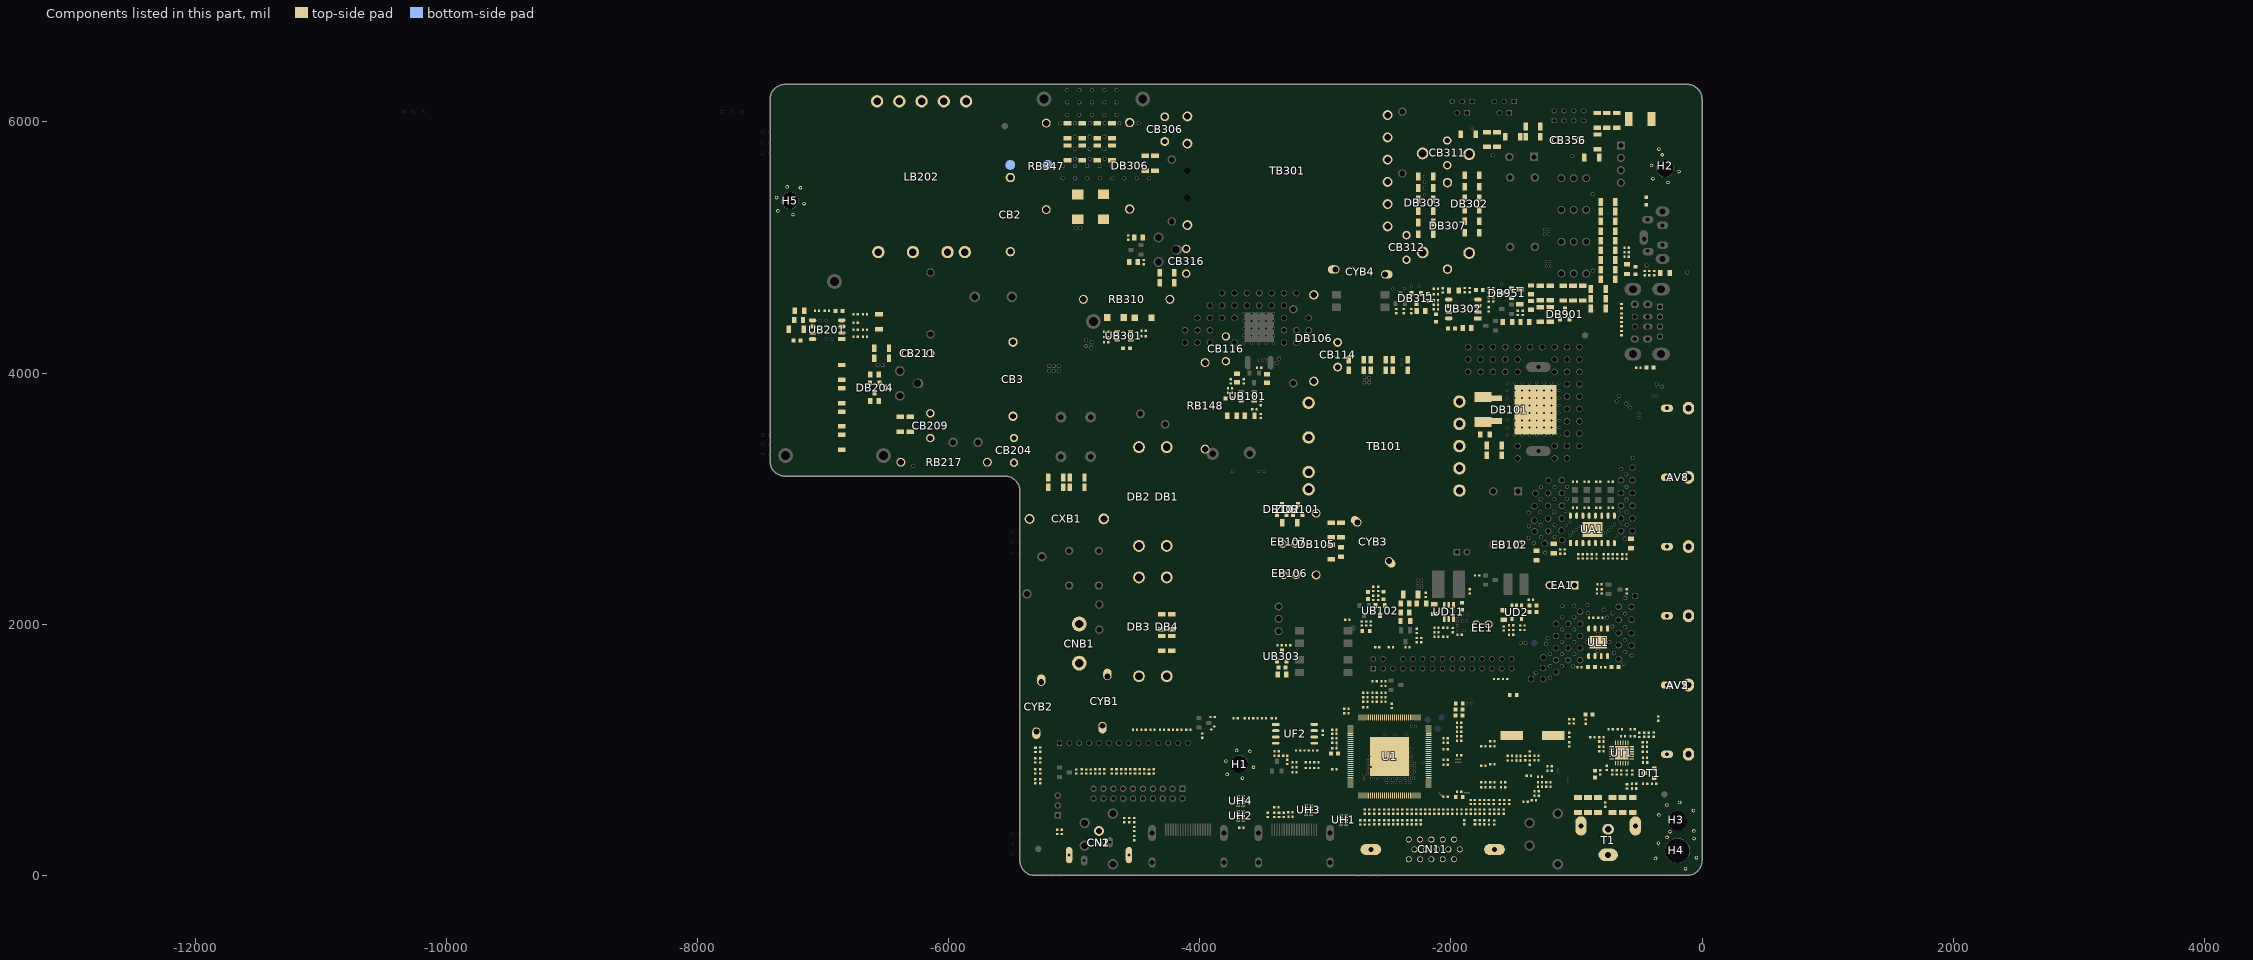
[diagram p0: the components of this part, seen from the top]
# Altium PCB MISC84277.PcbDoc (part 3 of 15)
Units mil, origin at the board's own origin, x right, y up, seen from the top; angles counter-clockwise.
Board outline 7422.08 x 6299.21 mil, 2 copper layers (TopLayer, BottomLayer), stack 61.855 mil thick; 709 components, 395 nets, 2812 pads, 811 vias.

## Components (designator, comment, footprint, x,y, rotation, side; value= is the part's Value field where it differs from the comment) (continued)
RB210 "10ohm-1206-±5%-1/4W" R1206 -7213.93,4349.5 r180 top
RB212 "47ohm-0805-±5%-1/8W" R0805 -6589.92,3989.81 r0 top
RB213 "20ohm-0805-±5%-1/8W" R0805 -6589.92,3777.97 r0 top
RB214 "10Kohm-0402-±5%-1/16W" R0402 -6502.12,3881.88 r90 top
RB215 "510ohm-0402-±5%-1/16W" R0402 -6666.39,4468.8 r0 top
RB217 "MOF-0R1ohm-±5%-2WS (tape and reel/Futaba)" R2-H-17.5 -6036.5,3290.5 r180 top
RB218 "1R6ohm-1206-±1%-1/4W" R1206 -6555,4409.94 r90 top
RB219 "22ohm-1206-±5%-1/4W" R1206 -6305.64,3592.04 r90 top
RB220 "22ohm-1206-±5%-1/4W" R1206 -6385.37,3592.04 r90 top
RB221 "1Kohm-0402-±5%-1/16W" R0402 -6666.39,4345.31 r180 top
RB223 "22ohm-1206-±5%-1/4W" R1206 -6534.37,4118.08 r180 top
RB224 "22ohm-1206-±5%-1/4W" R1206 -6534.37,4196.82 r180 top
RB225 "10Kohm-0402-±5%-1/16W" R0402 -6970.22,4496.35 r180 top
RB226 "47Kohm-0402-±1%-1/16W" R0402 -6741.19,4400.61 r180 top
RB227 "NC/0ohm-0402-±5%-1/16W" R0402 -7048.96,4496.35 r0 top
RB301 "47ohm-0805-±5%-1/8W" R0805 -1871,4360.5 r0 top
RB302 "8K2ohm-0402-±1%-1/16W" R0402 -3296.5,1832.5 r0 top
RB303 "NC/10Kohm-0402-±5%-1/16W" R0402 -4745.41,4244.24 r180 top
RB304 "47Kohm-0402-±1%-1/16W" R0402 -4447.08,4338.63 r0 top
RB305 "510ohm-0402-±5%-1/16W" R0402 -4745.41,4330.86 r180 top
RB306 "47ohm-0805-±5%-1/8W" R0805 -4489.97,5079.5 r0 top
RB307 "510ohm-0402-±5%-1/16W" R0402 -4569.47,5079.5 r270 top
RB308 "20ohm-0805-±5%-1/8W" R0805 -4527.5,4883.5 r0 top
RB309 "10Kohm-0402-±5%-1/16W" R0402 -4448,4883.5 r90 top
RB310 "MOF-0R22ohm-±5%-2WS (tape and reel/Futaba)" R2-H-17.5 -4582.61,4587.13 r180 top
RB314 "10ohm-1206-±5%-1/4W" R1206 -4435.6,5670.34 r270 top
RB315 "10ohm-1206-±5%-1/4W" R1206 -4356.88,5670.34 r270 top
RB317 "330Kohm-1206-±5%-1/4W" R1206 -4699.09,5753.57 r270 top
RB318 "330Kohm-1206-±5%-1/4W" R1206 -4817.2,5753.57 r270 top
RB319 "330Kohm-1206-±5%-1/4W" R1206 -4935.31,5753.57 r270 top
RB320 "330Kohm-1206-±5%-1/4W" R1206 -5053.42,5753.57 r270 top
RB321 "330Kohm-1206-±5%-1/4W" R1206 -5053.42,5930.74 r270 top
RB322 "330Kohm-1206-±5%-1/4W" R1206 -4699.09,5930.74 r270 top
RB323 "330Kohm-1206-±5%-1/4W" R1206 -4817.2,5930.74 r270 top
RB324 "330Kohm-1206-±5%-1/4W" R1206 -4935.31,5930.74 r270 top
RB325 "49K9ohm-0402-±1%-1/16W" R0402 -3364,1832.5 r180 top
RB326 "100ohm-0805-±5%-1/8W" R0805 -3345.5,1600 r0 top
RB328 "270Kohm-1206-±5%-1/4W" R1206 -1832.22,5484.11 r180 top
RB329 "270Kohm-1206-±5%-1/4W" R1206 -1832.22,5392.31 r0 top
RB330 "270Kohm-1206-±5%-1/4W" R1206 -1832.22,5116.9 r180 top
RB331 "270Kohm-1206-±5%-1/4W" R1206 -2200.06,5198.86 r180 top
RB332 "NC/270Kohm-1206-±5%-1/4W" R1206 -1832.22,5575.91 r180 top
RB333 "NC/270Kohm-1206-±5%-1/4W" R1206 -1832.22,5300.5 r0 top
RB334 "NC/270Kohm-1206-±5%-1/4W" R1206 -1832.22,5208.7 r180 top
RB335 "NC/270Kohm-1206-±5%-1/4W" R1206 -2200.06,5107.06 r180 top
RB337 "1R6ohm-1206-±1%-1/4W" R1206 -879.7,5717.5 r0 top
RB338 "1R6ohm-1206-±1%-1/4W" R1206 -833.45,5841.2 r270 top
RB339 "1R6ohm-1206-±1%-1/4W" R1206 -680.42,6012.54 r90 top
RB340 "1R6ohm-1206-±1%-1/4W" R1206 -758.2,6012.55 r90 top
RB341 "2R2ohm-1206-±1%-1/4W" R1206 -835.79,6012.54 r90 top
RB345 "5K6ohm-0402-±1%-1/16W" R0402 -2065.5,4659 r270 top
RB346 "510ohm-0402-±5%-1/16W" R0402 -2435,4493.5 r90 top
RB347 "NC/MOF-300Kohm-±5%-2WS (tape and reel/Futaba)" R2-H-17.5 -5223,5646.5 r270 top
RB348 "1Kohm-0402-±5%-1/16W" R0402 -2120.5,4508 r0 top
RB349 "27Kohm-0402-±1%-1/16W" R0402 -2120.5,4544.5 r180 top
RB350 "1Kohm-0603-±1%-1/10W" R0603 -2119.5,4437.5 r270 top
RB351 "10Kohm-0402-±5%-1/16W" R0402 -2120.57,4673.43 r0 top
RB352 "NC/20Kohm-0402-±1%-1/16W" R0402 -1850.5,4660.5 r270 top
RB354 "3Kohm-0402-±1%-1/16W" R0402 -1700,4507 r270 top
RB355 "4K7ohm-0402-±1%-1/16W" R0402 -1662.85,4587.77 r90 top
RB356 "2M2ohm-0402-±5%-1/16W" R0402 -2318,4493.5 r270 top
RB357 "3Kohm-0402-±1%-1/16W" R0402 -1699.45,4658.94 r90 top
RB358 "120Kohm-0805-±5%-1/8W" R0805 -1363,4663.5 r270 top (schematic designator RB364)
RB359 "120Kohm-0805-±5%-1/8W" R0805 -1363,4540 r270 top
RB360 "150Kohm-1206-±5%-1/4W" R1206 -1288.48,4637.59 r90 top
RB361 "150Kohm-1206-±5%-1/4W" R1206 -1209.74,4466.73 r90 top
RB362 "150Kohm-1206-±5%-1/4W" R1206 -1288.48,4466.73 r90 top
RB363 "150Kohm-1206-±5%-1/4W" R1206 -1209.74,4637.59 r90 top
RB364 "30Kohm-0805-±1%-1/8W" R0805 -1412,4407.5 r180 top
RB365 "10ohm-0805-±5%-1/8W" R0805 -2237.5,4493 r0 top
RB366 "47Kohm-0402-±1%-1/16W" R0402 -1889,4660.5 r270 top
RB367 "1Kohm-0402-±5%-1/16W" R0402 -1662.84,4658.94 r90 top
RB368 "68ohm-1206-±5%-1/4W" R1206 -2200.06,5290.66 r180 top
RB369 "68ohm-1206-±5%-1/4W" R1206 -2200.06,5382.46 r180 top
RB370 "68ohm-1206-±5%-1/4W" R1206 -2200.06,5474.26 r180 top
RB371 "68ohm-1206-±5%-1/4W" R1206 -2200.06,5566.07 r180 top
RB384 "1Kohm-0603-±1%-1/10W" R0603 -2675.28,1944.88 r180 top
RB385 "4K7ohm-0402-±1%-1/16W" R0402 -2675.28,2005.98 r90 top
RB386 "9K1ohm-0402-±1%-1/16W" R0402 -2711.79,2005.98 r270 top
RB391 "22ohm-1206-±5%-1/4W" R1206 -4261.46,4798.93 r180 top
RB392 "22ohm-1206-±5%-1/4W" R1206 -4261.32,4720.7 r180 top
RB901 "NC/470ohm-1206-±5%-1/4W" R1206 -1028.31,4637.19 r270 top
RB902 "NC/470ohm-1206-±5%-1/4W" R1206 -1105.54,4637.19 r270 top
RB903 "NC/470ohm-1206-±5%-1/4W" R1206 -951.09,4637.19 r270 top
RB904 "0ohm-1206-±5%-1/4W" R1206 -1346.23,5881.2 r0 top
RB905 "NC/0ohm-1206-±5%-1/4W" R1206 -1346.23,5963.8 r0 top
RB911 "NC/10ohm-1206-±5%-1/4W" R1206 -749.28,5130.73 r180 top
RB912 "NC/10ohm-1206-±5%-1/4W" R1206 -749.28,5054.26 r180 top
RB913 "NC/10ohm-1206-±5%-1/4W" R1206 -749.28,4977.39 r180 top
RB921 "NC/10ohm-1206-±5%-1/4W" R1206 -749.28,5363.12 r180 top
RB922 "NC/10ohm-1206-±5%-1/4W" R1206 -749.28,5286.45 r180 top
RB923 "NC/10ohm-1206-±5%-1/4W" R1206 -749.28,5209.28 r180 top
RB931 "NC/10ohm-1206-±5%-1/4W" R1206 -827.49,4670.39 r180 top
RB932 "NC/10ohm-1206-±5%-1/4W" R1206 -827.49,4592.62 r180 top
RB933 "NC/10ohm-1206-±5%-1/4W" R1206 -827.49,4514.85 r180 top
RB941 "NC/10ohm-1206-±5%-1/4W" R1206 -749.28,4900.13 r180 top
RB942 "NC/10ohm-1206-±5%-1/4W" R1206 -749.18,4823.97 r180 top
RB943 "NC/10ohm-1206-±5%-1/4W" R1206 -749.28,4748.1 r180 top
RB951 "NC/2Kohm-0402-±1%-1/16W" R0402 -1469.49,4480.1 r90 top
RB952 "NC/20Kohm-1206-±5%-1/4W" R1206 -1452.6,4608.64 r90 top
RD1 "100Kohm-0402-±1%-1/16W" R0402 -2115,1973 r0 top
RD6 "12K4ohm-0402-±1%-1/16W" R0402 -1520,1954 r180 top
RD7 "13Kohm-0402-±1%-1/16W" R0402 -1520,1991 r0 top
RD8 "68Kohm-0402-±1%-1/16W" R0402 -1431,1954 r0 top
RD12 "18Kohm-0402-±1%-1/16W" R0402 -2044,1900 r0 top
RD13 "100Kohm-0402-±1%-1/16W" R0402 -2115,1936 r0 top
RD15 "22ohm-0402-±5%-1/16W" R0402 -1984.25,1952.76 r270 top
RD16 "3K3ohm-0402-±1%-1/16W" R0402 -2115,1900 r0 top
RF1 "NC/1Mohm-0402-±5%-1/16W" R0402 -1742,1026.8 r180 top
RF2 "10Kohm-0402-±5%-1/16W" R0402 -3489,1251 r180 top
RF3 "4K7ohm-0402-±5%-1/16W" R0402 -3411,1251 r180 top
RF8 "4K7ohm-0402-±5%-1/16W" R0402 -2833,1291 r180 top
RF9 "4K7ohm-0402-±5%-1/16W" R0402 -2833,1327 r180 top
RF10 "100ohm-0402-±5%-1/16W" R0402 -2572,508 r270 top
RF11 "100ohm-0402-±5%-1/16W" R0402 -2722,422 r270 top
RF12 "68ohm-0402-±5%-1/16W" R0402 -1916,507 r90 top
RF13 "4K7ohm-0402-±5%-1/16W" R0402 -2608,1381 r180 top
RF14 "200Kohm-0402-±5%-1/16W" R0402 -1291,784 r0 top
RF15 "200Kohm-0402-±5%-1/16W" R0402 -1214,870 r0 top
RF16 "68ohm-0402-±5%-1/16W" R0402 -2423,508 r90 top
RF18 "4K7ohm-0402-±5%-1/16W" R0402 -2682,1381 r180 top
RF19 "68ohm-0402-±5%-1/16W" R0402 -2168,507 r270 top
RG1 "510ohm-0402-±5%-1/16W" R0402 -2682,1417 r0 top
RG2 "0ohm-0402-±5%-1/16W" R0402 -2608,1417 r180 top
RH1 "10Kohm-0402-±5%-1/16W" R0402 -4479.9,828.18 r90 top
RH2 "10Kohm-0402-±5%-1/16W" R0402 -4441.8,828.18 r90 top
RH3 "22ohm-0402-±5%-1/16W" R0402 -4367.2,828.18 r90 top
RH4 "22ohm-0402-±5%-1/16W" R0402 -4553.4,828.18 r90 top
RH5 "1Kohm-0402-±5%-1/16W" R0402 -4867.9,827.4 r270 top
RH6 "10Kohm-0402-±5%-1/16W" R0402 -4904,826.9 r90 top
RH7 "10Kohm-0402-±5%-1/16W" R0402 -4985.1,826.9 r90 top
RH8 "10Kohm-0402-±5%-1/16W" R0402 -3139.7,899.9 r0 top
RH9 "10Kohm-0402-±5%-1/16W" R0402 -3246.3,899.9 r180 top
RH10 "22ohm-0402-±5%-1/16W" R0402 -3072.4,855.1 r180 top
RH11 "22ohm-0402-±5%-1/16W" R0402 -3072.4,899.9 r180 top
RH13 "220ohm-0402-±5%-1/16W" R0402 -3139.7,855.1 r180 top
RH14 "1Kohm-0402-±5%-1/16W" R0402 -3319.7,953.77 r0 top
RH15 "10Kohm-0402-±5%-1/16W" R0402 -3246.3,823 r0 top
RH16 "10Kohm-0402-±5%-1/16W" R0402 -3246.3,860 r0 top
RH19 "NC/NC/100ohm-0402-±5%-1/16W" R0402 -3388.3,989.7 r180 top
RH20 "NC/NC/100ohm-0402-±5%-1/16W" R0402 -3388.3,954 r180 top
RH55 "NC/33Kohm-0402-±5%-1/16W" R0402 -4795.5,828.1 r270 top
RH56 "NC/22Kohm-0402-±5%-1/16W" R0402 -4759.7,828.2 r270 top
RI1 "NC/0ohm-0402-±5%-1/16W" R0402 -1734,423 r270 top
RI2 "0ohm-0402-±5%-1/16W" R0402 -1734,507 r270 top
RI3 "33ohm-0402-±5%-1/16W" R0402 -2024,507 r270 top
RI4 "10Kohm-0402-±5%-1/16W" R0402 -1692,507 r270 top
RI5 "12Kohm-0402-±5%-1/16W" R0402 -1809,584 r270 top
RI6 "10Kohm-0402-±5%-1/16W" R0402 -1698,584 r90 top
RI7 "12Kohm-0402-±5%-1/16W" R0402 -1735,584 r90 top
RI8 "10Kohm-0402-±5%-1/16W" R0402 -1224,743 r0 top
RI9 "12Kohm-0402-±5%-1/16W" R0402 -1291,743 r0 top
RI10 "10Kohm-0402-±5%-1/16W" R0402 -1224,707 r0 top
RI11 "12Kohm-0402-±5%-1/16W" R0402 -1291,707 r180 top
RI12 "33ohm-0402-±5%-1/16W" R0402 -2242,508 r90 top
RI13 "75ohm-0402-±5%-1/16W" R0402 -2242,423 r90 top
RI14 "NC/33ohm-0402-±5%-1/16W" R0402 -2314,423 r270 top
RI15 "NC/75ohm-0402-±5%-1/16W" R0402 -2278,423 r270 top
RI16 "NC/33ohm-0402-±5%-1/16W" R0402 -2096,507 r270 top
RI17 "NC/75ohm-0402-±5%-1/16W" R0402 -1895,423 r270 top
RI18 "75ohm-0402-±5%-1/16W" R0402 -1697,422 r90 top
RK1 "22ohm-0402-±5%-1/16W" R0402 -3897.08,1173.56 r225 top
RK2 "1Kohm-0402-±5%-1/16W" R0402 -3897.5,1261.1 r0 top
RK3 "1Kohm-0402-±5%-1/16W" R0402 -3626,1251 r0 top
RK4 "4K7ohm-0402-±1%-1/16W" R0402 -3557,1251 r0 top
RK5 "510ohm-0402-±1%-1/16W" R0402 -5271.45,1001.36 r270 top
RK6 "680ohm-0402-±1%-1/16W" R0402 -5308.96,749.44 r90 top
RK7 "1Kohm-0402-±1%-1/16W" R0402 -5271.45,749.44 r90 top
RK8 "1K2ohm-0402-±1%-1/16W" R0402 -5271.45,828.18 r90 top
RK9 "2K2ohm-0402-±1%-1/16W" R0402 -5308.96,828.18 r90 top
RK10 "4K7ohm-0402-±1%-1/16W" R0402 -5271.45,916.17 r90 top
RK11 "15Kohm-0402-±1%-1/16W" R0402 -5308.96,916.17 r90 top
RK15 "4K7ohm-0402-±5%-1/16W" R0402 -4516.1,1160 r0 top
RK16 "1Kohm-0402-±5%-1/16W" R0402 -4448.3,1160 r180 top
RK18 "33Kohm-0402-±5%-1/16W" R0402 -2537,1381 r0 top
RK20 "10Kohm-0402-±5%-1/16W" R0402 -4162.6,1160 r180 top
RK21 "510ohm-0402-±5%-1/16W" R0402 -4230.6,1160 r180 top
RM1 "4K7ohm-0402-±5%-1/16W" R0402 -837,2262 r270 top
RM2 "200Kohm-0402-±1%-1/16W" R0402 -817,2317 r0 top
RM3 "10Kohm-0402-±5%-1/16W" R0402 -2537,1417 r180 top
RM4 "4K7ohm-0402-±5%-1/16W" R0402 -1791,2388 r180 top
RM5 "4K7ohm-0402-±5%-1/16W" R0402 -2235,1874 r90 top
RM6 "NC/4K7ohm-0402-±5%-1/16W" R0402 -2478,1817 r0 top
RM7 "47Kohm-0402-±1%-1/16W" R0402 -2272,1874 r90 top
RM8 "4K7ohm-0402-±5%-1/16W" R0402 -2608,1545 r0 top
RM10 "2K2ohm-0402-±5%-1/16W" R0402 -2537,1545 r0 top
RO1 "NC/510ohm-0402-±5%-1/16W" R0402 -1537,584 r270 top
RO2 "NC/0ohm-0402-±5%-1/16W" R0402 -1771,507 r90 top
RO3 "NC/47Kohm-0402-±5%-1/16W" R0402 -4522.89,369.5 r270 top
RO5 "NC/510ohm-0402-±5%-1/16W" R0402 -1581,508 r270 top
RO6 "0ohm-0402-±5%-1/16W" R0402 -4603.2,439.7 r90 top
RO7 "NC/47Kohm-0402-±5%-1/16W" R0402 -4563.06,439.7 r90 top
RO9 "NC/220ohm-0402-±5%-1/16W" R0402 -3150,994.42 r180 top
RO10 "NC/100ohm-0402-±5%-1/16W" R0402 -3217.4,994.42 r180 top
RO12 "75ohm-0402-±5%-1/16W" R0402 -1844,507 r270 top
RO13 "0ohm-0402-±5%-1/16W" R0402 -1808,507 r90 top
RO15 "NC/0ohm-0402-±5%-1/16W" R0402 -1655,507 r90 top
RO16 "NC/0ohm-0402-±5%-1/16W" R0402 -1771,423 r270 top
RO17 "NC/0ohm-0402-±5%-1/16W" R0402 -1610,584 r270 top
RT1 "0ohm-0402-±5%-1/16W" L0402 -1462.17,951.3 r180 top
RT2 "100ohm-0402-±5%-1/16W" R0402 -802.35,1025.41 r0 top
RT3 "4K7ohm-0402-±5%-1/16W" R0402 -1059.05,1227.1 r270 top
RT4 "4K7ohm-0402-±5%-1/16W" R0402 -1021.7,1227.1 r270 top
RT5 "33ohm-0402-±5%-1/16W" R0402 -422.97,1119.86 r270 top
RT6 "33ohm-0402-±5%-1/16W" R0402 -385.62,1120.41 r270 top
RT7 "FCM1005KF-121T06(120ohm-500mA)" R0402 -928.4,1224.4 r270 top
RT9 "220ohm-0402-±5%-1/16W" R0402 -1318.94,950.79 r0 top
RT10 "220ohm-0402-±5%-1/16W" R0402 -1318.94,915.79 r0 top
RT11 "1K8ohm-0402-±5%-1/16W" R0402 -552.92,1107.68 r180 top
RT12 "430ohm-0402-±5%-1/16W" R0402 -1409.45,933.07 r90 top
RT14 "0ohm-0402-±5%-1/16W" L0402 -1462.17,914.8 r180 top
RT18 "10Kohm-0402-±5%-1/16W" R0402 -1670,885 r180 top
RU1 "5R1ohm-0402-±5%-1/16W" R0402 -1935,1178.5 r0 top
RU2 "5R1ohm-0402-±5%-1/16W" R0402 -1935,1107 r0 top
RU3 "5R1ohm-0402-±5%-1/16W" R0402 -1935,1214.5 r0 top
RU4 "5R1ohm-0402-±5%-1/16W" R0402 -1935,1143 r0 top
RV1 "33ohm-0402-±5%-1/16W" R0402 -2387,423 r270 top
RV2 "75ohm-0402-±5%-1/16W" R0402 -2350,423 r270 top
RV3 "33ohm-0402-±5%-1/16W" R0402 -2460,423 r270 top
RV4 "12Kohm-0402-±5%-1/16W" R0402 -1670,701.01 r180 top
RV5 "75ohm-0402-±5%-1/16W" R0402 -2423,423 r270 top
RV6 "10Kohm-0402-±5%-1/16W" R0402 -1585,701.01 r0 top
RV7 "10Kohm-0402-±5%-1/16W" R0402 -1585,740 r0 top
RV8 "12Kohm-0402-±5%-1/16W" R0402 -1670,740 r0 top
RV9 "33ohm-0402-±5%-1/16W" R0402 -2532,423 r270 top
RV10 "100ohm-0402-±5%-1/16W" R0402 -2649,422 r90 top
RV11 "75ohm-0402-±5%-1/16W" R0402 -2496,423 r270 top
RV12 "100ohm-0402-±5%-1/16W" R0402 -2610,423 r90 top
RV13 "10Kohm-0402-±5%-1/16W" R0402 -2572,423 r90 top
RV14 "10Kohm-0402-±5%-1/16W" R0402 -2685,422 r90 top
S/N1 "Barcode" Barcode -504.5,3364.84 r90 top
S/N2 "Barcode" BARCODE -1394,1364 r0 bottom
T1 "RF connector,RF JACK,H,IEC,T14.5,CH6.3,12.4×13.2×7.7mm,DIP,LHD-020 assembly,LHD" ANT-IEC14.5-H-短体-NG -748.03,153.7 r0 top locked
TB101 "SYEQ2612-T012A-YX" T/EQ2512*11 -2639,3418.5 r0 top locked
TB301 "SYEQ32 (large-size constant current)" T/EQ3214*11 -3144.5,5611.5 r180 top locked
TP-TDT "" TP-TDT -5362,5658.5 r180 bottom locked
U1 "TV main chip,IC Main Chip,TSUMV56RUU-Z1,32bit,Single-Core,QFP,SMD,Mstar" QFP128/0.4-5 -2489.44,946.68 r0 top locked
UA1 "Audio amplifier, IC Audio AMP, Class D, 2×13W@13V@8ohm, TSSOP-16, SMD, CSY1281AER, ON-Bright" SOP16/1.27-7 -874.02,2754.94 r90 top
UB101 "PWM controller, IC PWM Controller, 65KHZ, SOT23-6, SMD, OB2273C, ON-Bright" SOT-26 -3618.5,3814.5 r270 top locked
UB102 "AZ431AN-ATRE1(BCD)" SOT-23-RAK -2564.96,2108.27 r180 top
UB201 "PWM controller, IC PWM Controller, 300KHz, SOP-8, SMD, FAN7930CMX_G, Fairchild" SO-8A -6967.86,4345.37 r180 top
UB301 "PWM controller, IC PWM Controller, 65KHZ, SOT23-6, SMD, OB2273C, ON-Bright" SOT-26 -4605.04,4297.24 r270 top
UB302 "Operational amplifier, IC AMP, 2 channel, SOIC8, SMD, BA10358F-BZSE2, ROHM" SO-8A -1901.42,4511 r180 top locked
UB303 "AZ431AN-ATRE1(BCD)" SOT-23-RAK -3346.5,1745.47 r0 top
UD2 "LC2127CB5TR" SOT-23-5 -1476.7,2095.38 r180 top
UD11 "MP1470GJ-Z" SOT-23-6 -2016.7,2098.35 r180 top locked
UF2 "SPI FLASH chip, IC SPI FLASH, 32Mb, SOIC8, SMD, GD25Q32CSIG, GigaDevice" SOIC8 -3242,1127 r0 top
UH1 "NC/TVS diode, DIO ESD, 0.4pF, 19V, DFN2510-10L, SMD, ESD5304D-10/TR, Willsemi" RCL0524P -2855.5,441.3 r270 top
UH2 "NC/TVS diode, DIO ESD, 0.4pF, 19V, DFN2510-10L, SMD, ESD5304D-10/TR, Willsemi" RCL0524P -3675.07,473.17 r270 top
UH3 "NC/TVS diode, DIO ESD, 0.4pF, 19V, DFN2510-10L, SMD, ESD5304D-10/TR, Willsemi" RCL0524P -3134.17,521.1 r270 top
UH4 "NC/TVS diode, DIO ESD, 0.4pF, 19V, DFN2510-10L, SMD, ESD5304D-10/TR, Willsemi" RCL0524P -3675.07,592.32 r270 top
UL1 "LC1118CS8TR1833" SOP8/1.27-3 -828,1856 r270 top
UT1 "Silicon tuner, IC Si Tuner, QFN24, SMD, R842, Rafael" QFN24/0.5-3 -639.92,975.31 r180 top locked
XXXXXX "PCB_TIME" PCB_TIME -1322,1129 r90 top
XXXXXXXXXXXX "PCB_NAME" PCB_NAME -1560,1273 r90 top
YF1 "24MHz-±20PPM-20PF-HC-49S-SMD" XTAL-S-1 -1351,1114.26 r180 top
ZDB101 "BZX84C24 (Bluearrow)" SO-23 -3219,2915.5 r180 top
硅胶 "NC/glue, 0.1g, silicone" "HEAT-SHRINKABLE TUBE" -70,70 r90 top

## Footprints (in the part's own frame and the unit in brackets; to place one, negate y for a bottom-side part, rotate by r counter-clockwise, add the part's x,y. Pads: shape width x height; smd on the part's side, far side on the other; paste and mask are expansions set on the pad)
ANT-IEC14.5-H-短体-NG [mm] "RF-A814.5  短体 中心高度6.3mm 160323"
  oval 2.5x4.1 on Top Overlay paste-4 mask-4: 0(-5.5,6.1) 0(5.5,6.1)
  oval 4.1x2.7 on Top Overlay paste-4 mask-4: 0(0,0.25)
  oval 2.7x2.4 on Top Overlay: 0(0,5.45)
  oval 2.4x2.1 hole 1.3 slot 1.6 at 0 deg: 1(0,5.45)
  oval 2.3x3.9 hole 1 slot 2.6 at 90 deg: 2(-5.5,6.1) 4(5.5,6.1)
  oval 3.9x2.5 hole 1.2 slot 2.6 at 0 deg: 3(0,0.25)
  KeepOutLayer pour cut-out: -1.524,5.45 -1.395,4.889 -1.062,4.42 -0.574,4.115 -0.007,4.019 -0.007,4.019 0.593,4.093 1.118,4.391 1.49,4.867 1.651,5.45 1.651,5.45 1.49,6.032 1.118,6.509 0.593,6.807 -0.007,6.881 -0.007,6.881 -0.574,6.785 -1.062,6.48 -1.395,6.011 -1.524,5.45
  silkscreen extent -6.3,0 6.3,7.9
ASSE3.5C-3#1 [mm] "定位孔(顶底层上锡)"
  round 3.5 hole 3.5 unplated mask+0: 0(0,0)
  round 0.7 hole 0.4: 1(-2.464,-2.083) 2(-2.718,0.61) 3(-0.559,2.769) 4(2.108,2.591) 5(2.845,-0.635) 6(0.61,-2.845)
ASSE3.5C-3#2 [mm] "定位孔(顶底层上锡)"
  round 3.5 hole 3.5 unplated mask+0: 0(0,0)
  round 0.7 hole 0.4: 1(-2.464,-2.083) 2(-2.718,0.61) 3(-0.559,2.769) 4(-1.233,3.9) 5(2.845,-0.635) 6(0.61,-2.845)
ASSE4.0C-4 [mm] "定位孔(顶底层上锡)"
  round 4 hole 4 unplated mask+0: 0(0,0)
  round 0.7 hole 0.4: 1(-3.759,1.245) 2(-2.108,3.226) 3(0.457,3.734) 4(3.226,2.108) 5(3.327,-2.007) 6(-2.071,-3.302)
ASSE5.0C-4 [mm] "定位孔(顶底层上锡)"
  round 5 hole 5 unplated mask+0: 0(0,0)
  round 0.7 hole 0.4: 1(-4.394,-1.575) 2(-3.835,1.524) 3(-1.499,3.835) 4(3.378,2.43) 5(3.861,-1.422) 6(1.651,-3.658)
AV1-H-4 [mm] "强生；AV38A-01S-5020;中心高度为5.5mm;14.08.09"
  round 2 hole 1.2 mask+0.076: 1(0,8.05)
  round 2.2 on Top Overlay mask+0.076: 2(0,8.05)
  oval 1.3x3.3 hole 0.6 slot 2.6 at 90 deg mask+0.076: 2(6.05,3.15) 3(-6.05,3.15)
  oval 1.5x3.5 on Top Overlay mask+0.076: 3(-6.05,3.15) 3(6.05,3.15)
  silkscreen extent -6.4,0 6.4,8.7
AV3-H14-15 [mm] "宇球；RC075-F03L3BY-A; 中心高度：5.5mm;15.11.24;170401兼容物料，更新高度;170802加大接地脚焊盘（18.03.09更新孔距）"
  oval 2.8x2.5 on Top Overlay: 0(-14,2.75) 0(0,2.75) 0(14,2.75)
  oval 1.7x2.7 on Top Overlay: 0(-14,7.1) 0(0,7.1) 0(14,7.1)
  oval 1.5x2.5 hole 0.8 slot 1.8 at 90 deg: 1(-14,7.1) 3(0,7.1) 5(14,7.1)
  oval 2.6x2.3 hole 1.3 slot 1.6 at 0 deg: 2(-14,2.75) 4(0,2.75) 6(14,2.75)
  silkscreen extent -20.3,0 20.3,7.8, body extent -20.1,-9 20.1,7.9, height 10.7
Barcode [mil]
  silkscreen extent -576,-157 606,158
BARCODE [mil]
  silkscreen extent -576,-157 606,158
C0402 [mm] "片式电容"
  rect 0.45x0.5 smd mask+0.076: 1(-0.425,0) 2(0.425,0)
  silkscreen extent -0.88,-0.4 0.88,0.4, body extent -0.5,-0.25 0.5,0.25, height 0.5
C0603 [mm] "片式电容"
  rect 0.8x0.8 smd mask+0.076: 1(-0.706,0) 2(0.706,0)
  silkscreen extent -1.39,-0.55 1.39,0.55, body extent -0.8,-0.4 0.8,0.4, height 0.8
C0805 [mm] "片式电容"
  rect 0.9x1.25 smd mask+0.076: 1(-0.966,0) 2(0.966,0)
  silkscreen extent -1.73,-0.78 1.73,0.78, body extent -1,-0.62 1,0.63, height 1.25
C1206 [mm] "片式电容"
  rect 1x1.6 smd mask+0.076: 1(-1.5,-0.001) 2(1.5,0.001)
  silkscreen extent -2.39,-0.95 2.39,0.95, body extent -1.6,-0.8 1.6,0.8, height 1.3
CAP7.5*2.5-V-5 [mm] "同皓电子"
  round 1.7 hole 1.1: 1(-2.5,0) 2(2.5,0)
  round 1.9 on Top Overlay: 43(2.5,0) 44(-2.5,0)
  silkscreen extent -3.75,-1.25 3.75,1.25
CAP8*2.5-V-5 [mm] "C242G472J20A201(编带/法拉)"
  round 1.8 hole 1.1: 1(-2.5,0) 2(2.5,0)
  round 2 on Top Overlay: 1(-2.5,0) 1(2.5,0)
  silkscreen extent -4,-1.25 4,1.25
CAP8.5*4-V-5 [mm] "Walsin；LR102102K070BAND5B-低损(编带/Walsin);15.07.30/CT81-1KV-08b-HR-102K-T (12mm)"
  round 1.7 hole 1.1: 1(-2.5,0) 2(2.5,0)
  round 1.9 on Top Overlay: 3(-2.5,0) 4(2.5,0)
  silkscreen extent -4.25,-2 4.25,2, body extent -4,-2.03 4,1.97, height 12.18
CAP9.8*4-V-5 [mm] "SHM;DCH472M36Y5UN6FL5A0;15.09.06"
  round 1.7 hole 1.1: 1(-2.5,0) 2(2.5,0)
  round 1.9 on Top Overlay: 3(-2.5,0) 4(2.5,0)
  silkscreen extent -4.91,-2 4.9,2, body extent -5.49,-2.5 5.5,2.5, height 12.5
CAP13*4.5-V-10 [mm] "YP1AH681K080BAMD0B(Walsin)(18.01.12更新孔径）"
  oval 2.35x1.7 hole 1.2 copper offset -0.375,0: 1(-5,0.5)
  oval 2.35x1.7 hole 1.2 copper offset 0.375,0: 2(5,-0.5)
  oval 2.55x1.9 on Top Overlay: 61(-5,0.5) 61(5,-0.5)
  silkscreen extent -6.5,-2.25 6.5,2.25
CAP18*7-V-15 [mm] "MPX450K474(散装/日精)"
  round 1.9 hole 1.2: 1(-7.5,0) 2(7.5,0)
  round 2.1 on Top Overlay: 73(7.5,0) 74(-7.5,0)
  silkscreen extent -8.9,-3.5 8.9,3.5
CAP18*8.5-V-15 [mm] "PX334K3ID49H200D9R(凯励)(18.01.12更新孔径）"
  round 2.2 / inner round 2.2 / far side round 1.8 hole 1.4: 1(-7.5,0)
  round 2 hole 1.4: 2(7.5,0)
  round 2.4 on Top Overlay: 77(7.5,0) 78(-7.5,0)
  silkscreen extent -9,-4.45 9,4.45
CAUTION [mil]
  silkscreen extent -400,-146 486,161
COLD [mil]
CON2-H7.92 [mm]
  round 3 hole 1.7: 1(0,3.96) 3(0,-3.96)
  round 3.2 on Top Overlay: 109(0,3.96) 110(0,-3.96)
  silkscreen extent -12,-8.14 1.31,7.86
CQC [mil]
D1-H-12.5 [mm] "FR107 二极管与FR207 共用封装"
  round 2 on Top Overlay: 13(-6.25,0) 14(6.25,0)
  round 1.8 hole 1.3: A(-6.25,0) K(6.25,0)
  silkscreen extent -5.5,-1.65 5.6,1.65
D2-H-17.5 [mm] "GOOD-ARK;HER201G~HER208G;14-04-18"
  round 2.1 on Top Overlay: 15(-8.75,0) 16(8.75,0)
  round 1.9 hole 1.3: A(-8.75,0) K(8.75,0)
  silkscreen extent -7.5,-1.8 7.5,1.8
D2PAK3 [mm] "伟达电子；SFS1006G;增加TO-252兼容；160309"
  rect 2x3.4 smd paste-5 mask-5: 1(-2.54,-10.6) 3(2.54,-10.6)
  rect 1.143x2.794 smd: 1(-2.3,-8.15) 3(2.3,-8.15)
  rect 10x8.5 smd paste-11 mask-11: 2(0,0)
  rect 6x6 smd: 2(0,-0.95)
  silkscreen extent -5.79,-7.95 5.79,4.54, body extent -5.25,-11.89 5.25,3.8, height 4.7
D3-H-20 [mm] "肖特基二极管"
  round 2.6 on Top Overlay: 0(10,0) 1(-10,0)
  round 2.4 hole 1.6: A(-10,0) K(10,0)
  silkscreen extent -13,-2.6 13,2.6
DB15-HF-1 [mm] "兴万联电子：WLHD-051A"
  oval 4.4x2.4 on Top Overlay: 0(-12.5,5.227) 0(12.5,5.227)
  round 1.2 hole 0.9: 1(4.33,7.247) 2(2.04,7.247) 3(-0.25,7.247) 4(-2.54,7.247) 5(-4.83,7.247) 6(5.475,5.247) 7(3.185,5.247) 8(0.895,5.247) 9(-1.395,5.247) 10(-3.685,5.247) 11(4.33,3.247) 12(2.04,3.247) 13(-0.25,3.247) 14(-2.54,3.247) 15(-4.83,3.247)
  oval 4.2x2.2 hole 1 slot 3 at 0 deg: 16(-12.5,5.227) 17(12.5,5.227)
  round 1.5 on Top Overlay: 30(-4.83,3.247) 31(-2.54,3.247) 32(-0.25,3.247) 33(2.04,3.247) 34(4.33,3.247) 35(5.475,5.247) 36(3.185,5.247) 37(0.895,5.247) 38(-1.395,5.247) 39(-3.685,5.247) 40(-4.83,7.247) 41(-2.54,7.247) 42(-0.25,7.247) 43(2.04,7.247) 44(4.33,7.247)
  BottomLayer pour cut-out: -4.814,8.609 -4.814,5.885 -4.587,5.885 -4.443,5.742 -3.456,5.742 -3.175,5.461 -3.175,5.029 -3.454,4.75 -4.42,4.75 -4.56,4.609 -4.797,4.609 -4.83,4.576 -4.83,1.885 4.33,1.885 4.33,3.247 4.298,3.279 4.298,4.609 4.105,4.609 3.95,4.764 2.44,4.764 2.285,4.609 1.817,4.609 1.664,4.763 0.648,4.763 0.368,5.042 0.368,5.474 0.622,5.728 1.651,5.728 1.803,5.88 2.286,5.88 2.438,5.728 3.95,5.728 4.107,5.885 4.33,5.885 4.33,8.609
  silkscreen extent -15.59,0 15.59,9.48, body extent -15.43,-6 15.37,8.5, height 12.43
DIODE-S0402 [mm] "DVD上使用的ESD"
  rect 0.45x0.55 smd mask+0.051: A(-0.425,0) K(0.425,0)
  silkscreen extent -0.8,-0.43 0.91,0.43, body extent -0.5,-0.25 0.5,0.25, height 0.5
DIODE-S-2 [mm] "1N5819-SMA"
  rect 1.6x2.8 smd: A(-2.3,0) K(2.3,0)
  silkscreen extent -3.5,-1.6 3.7,1.61, body extent -2.6,-1.4 2.6,1.4, height 1.91
DIODE-S-14 [mm] "ROHM;FSL14"
  rect 1.3x1.35 smd: A(1.675,0) K(-1.675,0)
  silkscreen extent -1.55,-1 1.55,1, body extent -1.95,-1 1.95,1, height 1.08
DIODE-SMB-1 [mm] "CITC;SK52B--SK520B"
  rect 1.95x2.25 smd: A(2.525,0) K(-2.525,0)
  silkscreen extent -2.4,-2 2.4,2.77, body extent -2.65,-2 2.65,2, height 2.5
EC(5*11)-V-2.5 [mm] "机插2.5间距"
  round 1.8 on Top Overlay: 0(-1.25,0) 0(1.25,0)
  round 0.5 on Keep-Out: 0(0,-0.787)
  round 1.6 hole 1.1: 1(-1.25,0) 2(1.25,0)
  silkscreen extent -2.67,-2.67 3,2.67, body extent -2.48,-2.52 2.5,2.47, height 7
EC(6.3*11)-V-2.5#1 [mm] "机插2.5间距"
  round 0.5 on Keep-Out: 0(0,-0.889)
  round 1.6 hole 1.1: 1(-1.25,0) 2(1.25,0)
  round 1.8 on Top Overlay: 5(1.25,0) 6(-1.25,0)
  silkscreen extent -3.17,-3.17 3.51,3.17, body extent -3,-3 2.98,2.99, height 12
EC(6.3*11)-V-2.5#2 [mm] "机插2.5间距"
  round 0.5 on Keep-Out: 0(-0.587,1.44)
  round 1.6 hole 1.1: 1(-1.25,0) 2(1.25,0)
  round 1.8 on Top Overlay: 5(1.25,0) 6(-1.25,0)
  silkscreen extent -3.17,-3.17 3.51,3.17, body extent -3,-3 2.98,2.99, height 12
EC(8*11)-V-3.5 [mm]
  rect 1.6x1.6 hole 1: 1(-1.75,0)
  rect 1.8x1.8 on Top Overlay: 1(-1.75,0)
  round 1.8 on Top Overlay: 1(1.75,0)
  round 1.6 hole 1: 2(1.75,0)
  silkscreen extent -4.25,-4.25 4.45,4.25, body extent -3.98,-3.98 4.01,4.01, height 12.51
EC(10*12)-V-5 [mm] "机插5间距"
  rect 1.9x1.9 on Top Overlay: 0(-2.5,0)
  round 0.5 on Keep-Out: 0(-0.75,0)
  round 1.9 on Top Overlay: 0(2.5,0)
  rect 1.7x1.7 hole 1.1: 1(-2.5,0)
  round 1.7 hole 1.1: 2(2.5,0)
  silkscreen extent -5.25,-5.25 5.57,5.25, body extent -4.98,-4.99 5.01,4.99, height 12.01